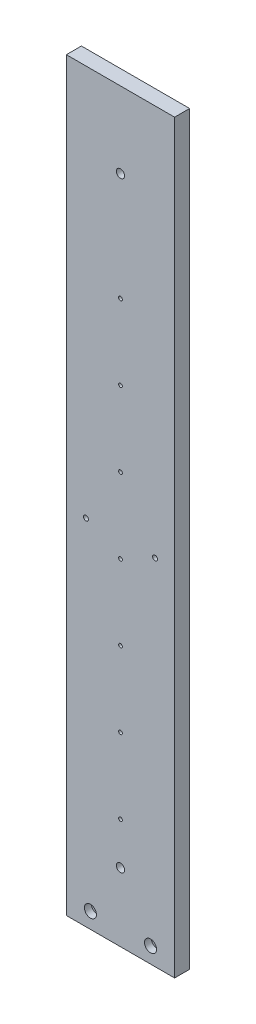
from build123d import *

# Parameters (mm, degrees)
SKETCH_1_W                = 72
SKETCH_1_H                = 496
EXTRUDE_1_DEPTH           = 10
HOLE_WIZARD_2_D           = 5.5
HOLE_WIZARD_2_CBORE_D     = 10
HOLE_WIZARD_2_CBORE_DEPTH = 5.7
HOLE_WIZARD_0_D           = 4.5
HOLE_WIZARD_0_CBORE_D     = 8
HOLE_WIZARD_0_CBORE_DEPTH = 4.6
HOLE_WIZARD_M4_2_D        = 3.3
HOLE_WIZARD_M4_2_DEPTH    = 10
HOLE_WIZARD_M4_2_TIP      = 0.991420021
HOLE_WIZARD_M4_3_D        = 3.3
HOLE_WIZARD_M3_1_D        = 2.5


with BuildPart() as part:
    # 草图1 → 凸台-拉伸1 (new body)
    with BuildSketch(Plane.XY):
        Rectangle(SKETCH_1_W, SKETCH_1_H)
    extrude(amount=EXTRUDE_1_DEPTH)

    # 打孔尺寸根据内六角圆柱头螺钉的类型2 (through all)
    with Locations(Plane(origin=(0, 0, 0), x_dir=(-1, 0, 0), z_dir=(0, 0, -1))):
        with Locations((0, -202.499999994), (0, 197.500000006)):
            CounterBoreHole(HOLE_WIZARD_2_D / 2, HOLE_WIZARD_2_CBORE_D / 2, HOLE_WIZARD_2_CBORE_DEPTH)

    # 打孔尺寸根据内六角圆柱头螺钉的类型0 (through all)
    with Locations(Plane.XY.offset(10)):
        with Locations((-20, -237.5), (20, -237.5)):
            CounterBoreHole(HOLE_WIZARD_0_D / 2, HOLE_WIZARD_0_CBORE_D / 2, HOLE_WIZARD_0_CBORE_DEPTH)

    # M4 螺纹孔2
    with Locations(Plane(origin=(0, -248, 0), x_dir=(-1, 0, 0), z_dir=(0, -1, 0))):
        with Locations((-12, -5), (-29, -5)):
            Hole(HOLE_WIZARD_M4_2_D / 2, depth=HOLE_WIZARD_M4_2_DEPTH)
            with Locations((0, 0, -(HOLE_WIZARD_M4_2_DEPTH + HOLE_WIZARD_M4_2_TIP / 2))):  # 118° drill point
                Cone(0, HOLE_WIZARD_M4_2_D / 2, HOLE_WIZARD_M4_2_TIP, mode=Mode.SUBTRACT)

    # M4 螺纹孔3 (through all)
    with Locations(Plane(origin=(0, 0, 0), x_dir=(-1, 0, 0), z_dir=(0, 0, -1))):
        with Locations((-23, -12.5), (23, -12.5)):
            Hole(HOLE_WIZARD_M4_3_D / 2)

    # M3 螺纹孔1 (through all)
    with Locations(Plane(origin=(0, 0, 0), x_dir=(-1, 0, 0), z_dir=(0, 0, -1))):
        with Locations((0, -174.5), (0, -124.5), (0, -74.5), (0, -24.5), (0, 25.5), (0, 75.5), (0, 125.5)):
            Hole(HOLE_WIZARD_M3_1_D / 2)


solid = part.part
